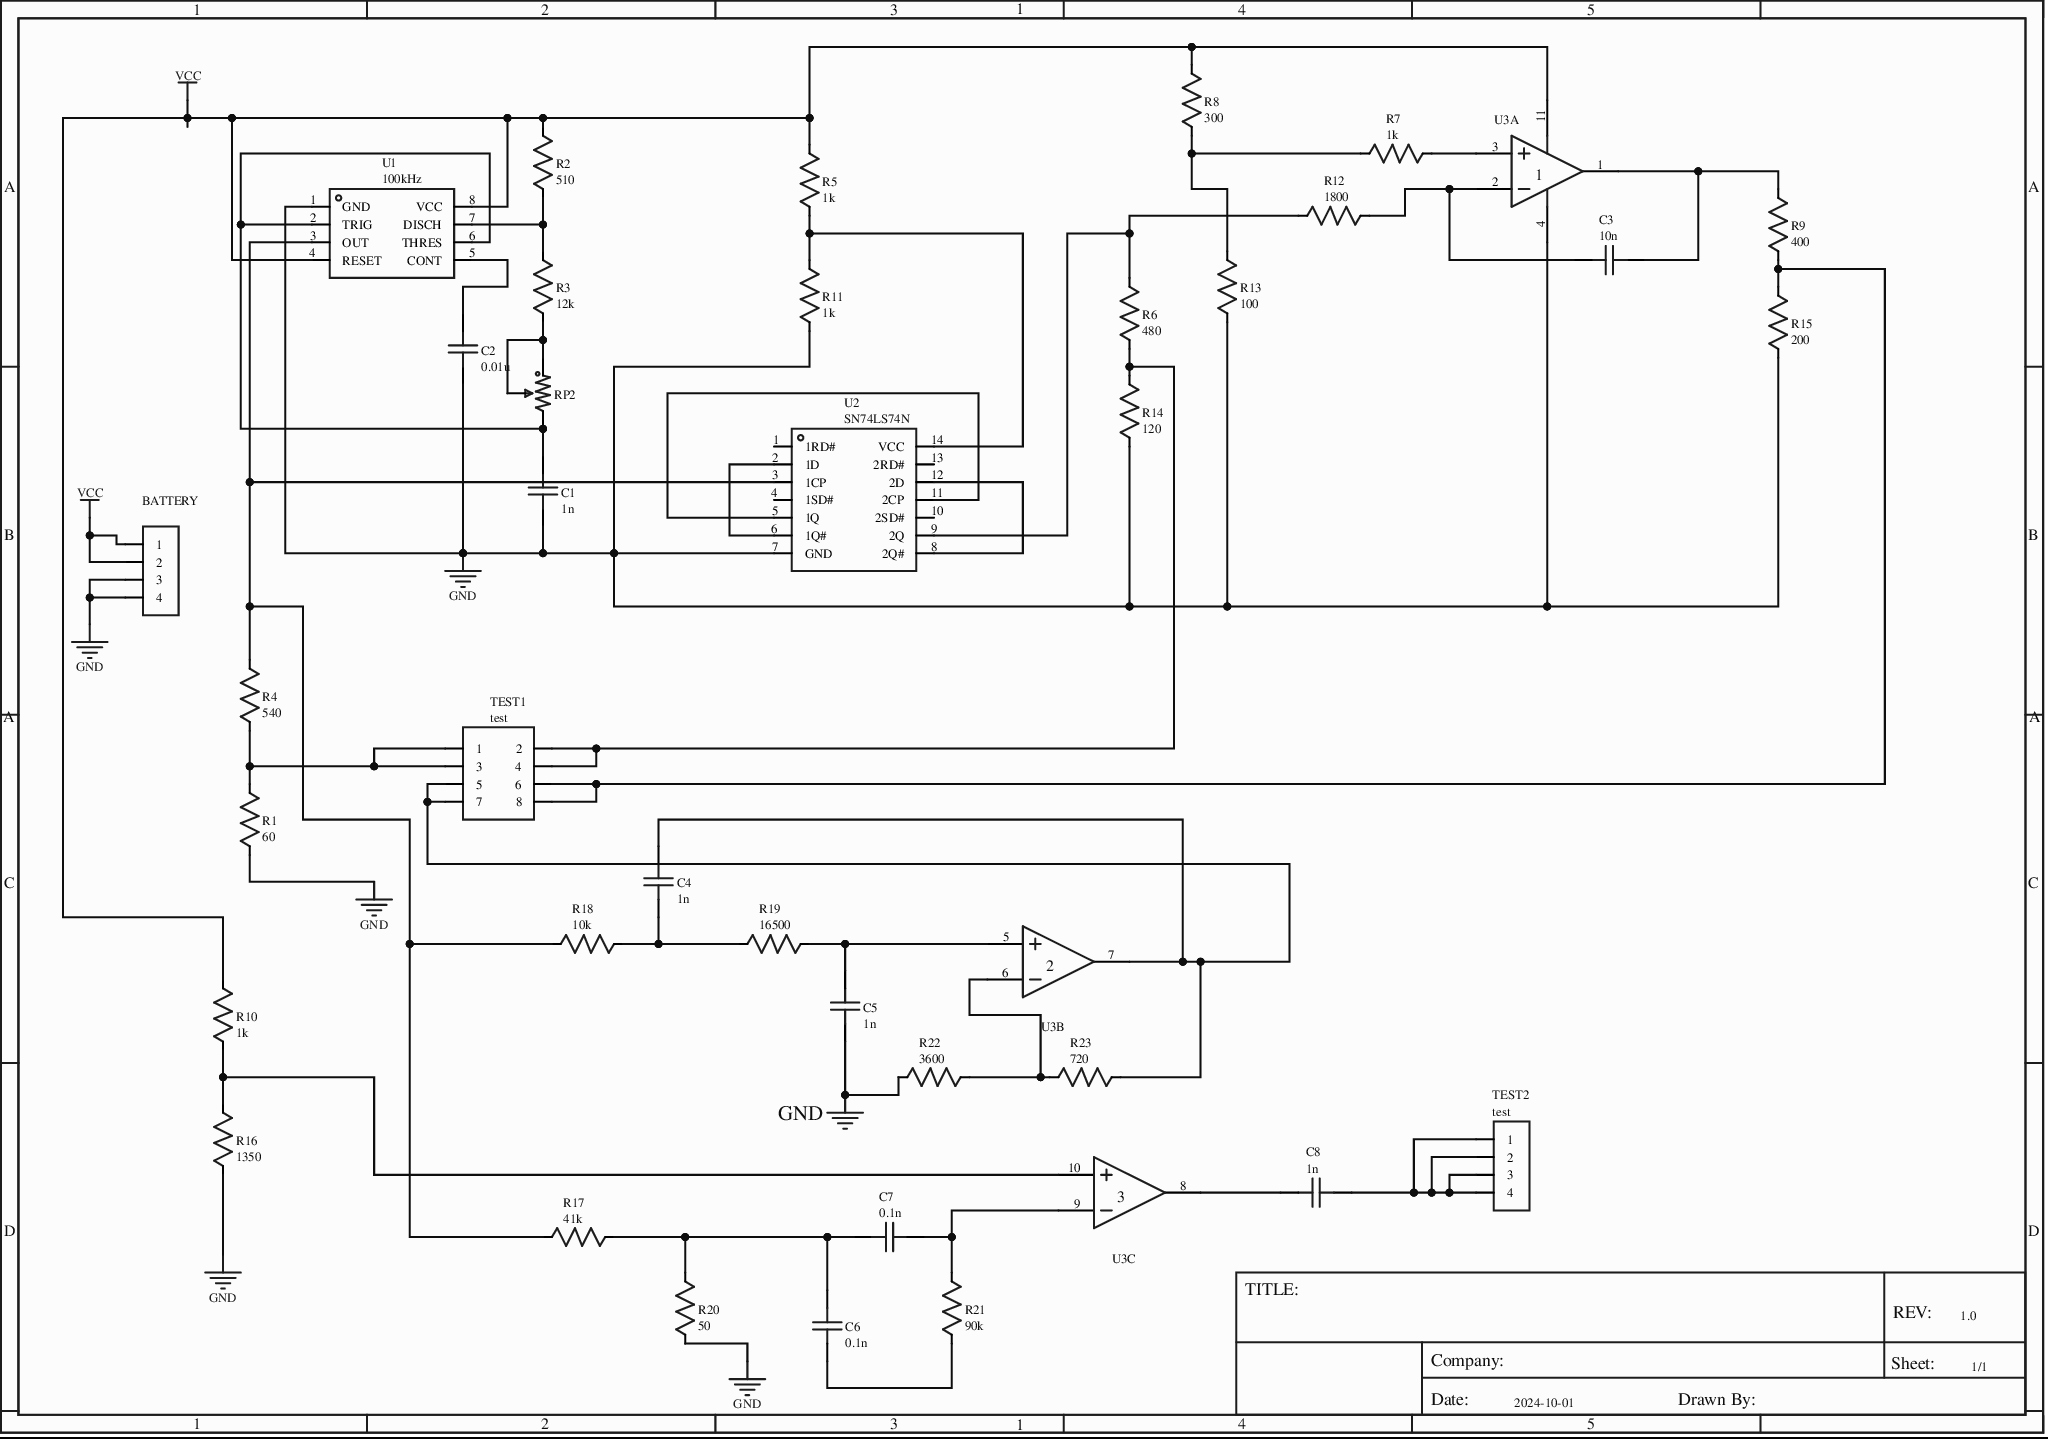
[diagram p0: MISC51938-3.schdoc]
# Altium project MISC51938-2.PrjPcb
1 sheet, 38 parts. Net scope: global (net labels, ports and power ports of the same name join across sheets).
Board file: MISC51938.pcbdoc

## Sheet MISC51938-3.schdoc
size 292 x 204 mm; Name: MISC51938; @Project Name: MISC51938; REV: 1.0; Date: 2024-10-01; Sheet: 1/1

### Parts
BATTERY  HDR-M-2.54_1x4  [HDR-M-2.54_1X4]  (value not drawn)
C1  1n  [RAD-0.1]
C2  0.01u  [RAD-0.1]
C3  10n  [RAD-0.1]
C4  1n  [RAD-0.1]
C5  1n  [RAD-0.1]
C6  0.1n  [RAD-0.1]
C7  0.1n  [RAD-0.1]
C8  1n  [RAD-0.1]
R1  60  [R_AXIAL-0.3]
R2  510  [R_AXIAL-0.3]
R3  12k  [R_AXIAL-0.3]
R4  540  [R_AXIAL-0.3]
R5  1k  [R_AXIAL-0.3]
R6  480  [R_AXIAL-0.3]
R7  1k  [R_AXIAL-0.3]
R8  300  [R_AXIAL-0.3]
R9  400  [R_AXIAL-0.3]
R10  1k  [R_AXIAL-0.3]
R11  1k  [R_AXIAL-0.3]
R12  1800  [R_AXIAL-0.3]
R13  100  [R_AXIAL-0.3]
R14  120  [R_AXIAL-0.3]
R15  200  [R_AXIAL-0.3]
R16  1350  [R_AXIAL-0.3]
R17  41k  [R_AXIAL-0.3]
R18  10k  [R_AXIAL-0.3]
R19  16500  [R_AXIAL-0.3]
R20  50  [R_AXIAL-0.3]
R21  90k  [R_AXIAL-0.3]
R22  3600  [R_AXIAL-0.3]
R23  720  [R_AXIAL-0.3]
RP2  R_3296W_US  [RES-ADJ-TH_3296W]  (value not drawn)
TEST1  test  [HDR-M-2.54_2X4]
TEST2  test  [HDR-M-2.54_1X4]
U1  100kHz  [DIP-8_L9.8-W6.6-P2.54-LS7.6-BL]
U2  SN74LS74N  [DIP-14_L19.1-W6.4-P2.54-LS7.6-BL]
U3  LM324_C5157701  [DIP-14_L18.9-W6.4-P2.54-LS7.6-BL]  (value not drawn)  (parts A,B,C of 3)

### Nets
GND: BATTERY.3 BATTERY.4 C1.1 C2.1 C5.1 R1.1 R11.1 R13.1 R14.1 R15.2 R16.1 R20.2 R22.2 U1.1(GND) U2.7(GND) U3.4(VCC)
VCC: BATTERY.1 BATTERY.2 R2.2 R5.2 R8.2 R10.2 U1.4(RESET) U1.8(VCC) U3.11(GND)
NetC1_2: C1.2 RP2.3 U1.2(TRIG) U1.6(THRES)
NetC2_2: C2.2 U1.5(CONT)
NetC3_1: C3.1 R9.1 U3.1(OUT1)
NetC3_2: C3.2 R12.1 U3.2(IN1-)
NetC4_1: C4.1 R18.1 R19.2
NetC4_2: C4.2 R23.1 TEST1.5 TEST1.7 U3.7(OUT2)
NetC5_2: C5.2 R19.1 U3.5(IN2+)
NetC6_1: C6.1 C7.1 R17.1 R20.1
NetC6_2: C6.2 R21.2
NetC7_2: C7.2 R21.1 U3.9(IN3-)
NetC8_1: C8.1 TEST2.1 TEST2.2 TEST2.3 TEST2.4
NetC8_2: C8.2 U3.8(OUT3)
NetR1_2: R1.2 R4.1 TEST1.1 TEST1.3
NetR2_1: R2.1 R3.2 U1.7(DISCH)
NetR3_1: R3.1 RP2.1 RP2.2
NetR4_2: R4.2 R17.2 R18.2 U1.3(OUT) U2.3(1CP)
NetR5_1: R5.1 R11.2 U2.14(VCC)
NetR6_1: R6.1 R14.2 TEST1.2 TEST1.4
NetR6_2: R6.2 R12.2 U2.9(2Q)
NetR7_1: R7.1 U3.3(IN1+)
NetR7_2: R7.2 R8.1 R13.2
NetR9_2: R9.2 R15.1 TEST1.6 TEST1.8
NetR10_1: R10.1 R16.2 U3.10(IN3+)
NetR22_1: R22.1 R23.2 U3.6(IN2-)
NetU2_2: U2.2(1D) U2.6(1Q#)
NetU2_5: U2.5(1Q) U2.11(2CP)
NetU2_8: U2.8(2Q#) U2.12(2D)

Not connected (* = marked no-connect by the designer): U2 1(1RD#)* 4(1SD#)* 10(2SD#)* 13(2RD#)*

### Notes on the sheet
- GND
- 1
- 2
- 3
- 4
- 5
- A
- B
- C
- D
- TITLE:
- Company:
- Sheet:
- REV:
- 1.0
- 1/1
- Date:
- 2024-10-01
- Drawn By:

### Library data of the parts
BATTERY = HDR-M-2.54_1x4: Convert to PCB: yes; UniqueId: gge182f55f181c338ac; ModelId: cd502121c3eb48dbbf0ecbc8e7ad097f; Origin Footprint: HDR-M-2.54_1X4; Device: HDR-M-2.54_1x4; Symbol: HDR-M-2.54_1x4; Supplier Part: C124378; Supplier: LCSC; Add into BOM: yes; FootprintName: HDR-M-2.54_1X4; ModelName: HDR-M-2.54_1x4
C1 = 1n: Convert to PCB: yes; UniqueId: ggebe2d0743338c48c7; ModelId: 1ae71cde80ce4853a0b9688090c601ad; ModelName: C_RAD-0.1; Origin Footprint: RAD-0.1; Device: 1n; Symbol: 1n; Add into BOM: yes; FootprintName: RAD-0.1
C2 = 0.01u: Convert to PCB: yes; UniqueId: ggec0655fcb97cffe8f; ModelId: 1ae71cde80ce4853a0b9688090c601ad; ModelName: C_RAD-0.1; Origin Footprint: RAD-0.1; Device: 0.01u; Symbol: 0.01u; Add into BOM: yes; FootprintName: RAD-0.1
C3 = 10n: Convert to PCB: yes; UniqueId: gge42024684f1aaf6c8; ModelId: 1ae71cde80ce4853a0b9688090c601ad; ModelName: C_RAD-0.1; Origin Footprint: RAD-0.1; Device: 10n; Symbol: 10n; Add into BOM: yes; FootprintName: RAD-0.1
C4 = 1n: Convert to PCB: yes; UniqueId: gge37dbe484222d80e1; ModelId: 1ae71cde80ce4853a0b9688090c601ad; ModelName: C_RAD-0.1; Origin Footprint: RAD-0.1; Device: 1n; Symbol: 1n; Add into BOM: yes; FootprintName: RAD-0.1
C5 = 1n: Convert to PCB: yes; UniqueId: gge837e8c776d9c40bf; ModelId: 1ae71cde80ce4853a0b9688090c601ad; ModelName: C_RAD-0.1; Origin Footprint: RAD-0.1; Device: 1n; Symbol: 1n; Add into BOM: yes; FootprintName: RAD-0.1
C6 = 0.1n: Convert to PCB: yes; UniqueId: gge8fb21ff73641724b; ModelId: 1ae71cde80ce4853a0b9688090c601ad; ModelName: C_RAD-0.1; Origin Footprint: RAD-0.1; Device: 0.1n; Symbol: 0.1n; Add into BOM: yes; FootprintName: RAD-0.1
C7 = 0.1n: Convert to PCB: yes; UniqueId: gge1a40875608363663; ModelId: 1ae71cde80ce4853a0b9688090c601ad; ModelName: C_RAD-0.1; Origin Footprint: RAD-0.1; Device: 0.1n; Symbol: 0.1n; Add into BOM: yes; FootprintName: RAD-0.1
C8 = 1n: Convert to PCB: yes; UniqueId: gge7d2a8f037e25720b; ModelId: 1ae71cde80ce4853a0b9688090c601ad; ModelName: C_RAD-0.1; Origin Footprint: RAD-0.1; Device: 1n; Symbol: 1n; Add into BOM: yes; FootprintName: RAD-0.1
R1 = 60: Convert to PCB: yes; UniqueId: gge0dfbe59a243fd0c6; ModelId: 3f997efe3b344f2d8e0a2d7f24a0763d; Origin Footprint: R_AXIAL-0.3; Device: 60; Symbol: 60; Add into BOM: yes; FootprintName: R_AXIAL-0.3; ModelName: R_AXIAL-0.3
R2 = 510: Convert to PCB: yes; UniqueId: ggef3c2f23d8da5d148; ModelId: 3f997efe3b344f2d8e0a2d7f24a0763d; Origin Footprint: R_AXIAL-0.3; Device: 510; Symbol: 510; Add into BOM: yes; FootprintName: R_AXIAL-0.3; ModelName: R_AXIAL-0.3
R3 = 12k: Convert to PCB: yes; UniqueId: gge48febd318e5da6c3; ModelId: 3f997efe3b344f2d8e0a2d7f24a0763d; Origin Footprint: R_AXIAL-0.3; Device: 12k; Symbol: 12k; Add into BOM: yes; FootprintName: R_AXIAL-0.3; ModelName: R_AXIAL-0.3
R4 = 540: Convert to PCB: yes; UniqueId: ggefea46ed2f578d9fb; ModelId: 3f997efe3b344f2d8e0a2d7f24a0763d; Origin Footprint: R_AXIAL-0.3; Device: 540; Symbol: 540; Add into BOM: yes; FootprintName: R_AXIAL-0.3; ModelName: R_AXIAL-0.3
R5 = 1k: Convert to PCB: yes; UniqueId: gge40155cd87b47f87c; ModelId: 3f997efe3b344f2d8e0a2d7f24a0763d; Origin Footprint: R_AXIAL-0.3; Device: 1k; Symbol: 1k; Add into BOM: yes; FootprintName: R_AXIAL-0.3; ModelName: R_AXIAL-0.3
R6 = 480: Convert to PCB: yes; UniqueId: ggef7fee3df49b55766; ModelId: 3f997efe3b344f2d8e0a2d7f24a0763d; Origin Footprint: R_AXIAL-0.3; Device: 480; Symbol: 480; Add into BOM: yes; FootprintName: R_AXIAL-0.3; ModelName: R_AXIAL-0.3
R7 = 1k: Convert to PCB: yes; UniqueId: ggef523a0c6794fa5f8; ModelId: 3f997efe3b344f2d8e0a2d7f24a0763d; Origin Footprint: R_AXIAL-0.3; Device: 1k; Symbol: 1k; Add into BOM: yes; FootprintName: R_AXIAL-0.3; ModelName: R_AXIAL-0.3
R8 = 300: Convert to PCB: yes; UniqueId: gge19ed68c85dd61d5f; ModelId: 3f997efe3b344f2d8e0a2d7f24a0763d; Origin Footprint: R_AXIAL-0.3; Device: 300; Symbol: 300; Add into BOM: yes; FootprintName: R_AXIAL-0.3; ModelName: R_AXIAL-0.3
R9 = 400: Convert to PCB: yes; UniqueId: gge2309c8064b6c3153; ModelId: 3f997efe3b344f2d8e0a2d7f24a0763d; Origin Footprint: R_AXIAL-0.3; Device: 400; Symbol: 400; Add into BOM: yes; FootprintName: R_AXIAL-0.3; ModelName: R_AXIAL-0.3
R10 = 1k: Convert to PCB: yes; UniqueId: gge1da9c41bb9003e75; ModelId: 3f997efe3b344f2d8e0a2d7f24a0763d; Origin Footprint: R_AXIAL-0.3; Device: 1k; Symbol: 1k; Add into BOM: yes; FootprintName: R_AXIAL-0.3; ModelName: R_AXIAL-0.3
R11 = 1k: Convert to PCB: yes; UniqueId: ggebda18a44617dddc0; ModelId: 3f997efe3b344f2d8e0a2d7f24a0763d; Origin Footprint: R_AXIAL-0.3; Device: 1k; Symbol: 1k; Add into BOM: yes; FootprintName: R_AXIAL-0.3; ModelName: R_AXIAL-0.3
R12 = 1800: Convert to PCB: yes; UniqueId: ggea9de047fd16be48d; ModelId: 3f997efe3b344f2d8e0a2d7f24a0763d; Origin Footprint: R_AXIAL-0.3; Device: 1800; Symbol: 1800; Add into BOM: yes; FootprintName: R_AXIAL-0.3; ModelName: R_AXIAL-0.3
R13 = 100: Convert to PCB: yes; UniqueId: gge3a1cc0d0732c84e9; ModelId: 3f997efe3b344f2d8e0a2d7f24a0763d; Origin Footprint: R_AXIAL-0.3; Device: 100; Symbol: 100; Add into BOM: yes; FootprintName: R_AXIAL-0.3; ModelName: R_AXIAL-0.3
R14 = 120: Convert to PCB: yes; UniqueId: ggec4de3e0c062074b8; ModelId: 3f997efe3b344f2d8e0a2d7f24a0763d; Origin Footprint: R_AXIAL-0.3; Device: 120; Symbol: 120; Add into BOM: yes; FootprintName: R_AXIAL-0.3; ModelName: R_AXIAL-0.3
R15 = 200: Convert to PCB: yes; UniqueId: gge992ac05409ed4dfa; ModelId: 3f997efe3b344f2d8e0a2d7f24a0763d; Origin Footprint: R_AXIAL-0.3; Device: 200; Symbol: 200; Add into BOM: yes; FootprintName: R_AXIAL-0.3; ModelName: R_AXIAL-0.3
R16 = 1350: Convert to PCB: yes; UniqueId: gge34052e6bc059f6cc; ModelId: 3f997efe3b344f2d8e0a2d7f24a0763d; Origin Footprint: R_AXIAL-0.3; Device: 1350; Symbol: 1350; Add into BOM: yes; FootprintName: R_AXIAL-0.3; ModelName: R_AXIAL-0.3
R17 = 41k: Convert to PCB: yes; UniqueId: ggec6451f7b0751eb53; ModelId: 3f997efe3b344f2d8e0a2d7f24a0763d; Origin Footprint: R_AXIAL-0.3; Device: 41k; Symbol: 41k; Add into BOM: yes; FootprintName: R_AXIAL-0.3; ModelName: R_AXIAL-0.3
R18 = 10k: Convert to PCB: yes; UniqueId: ggeadda2c91ca372ec2; ModelId: 3f997efe3b344f2d8e0a2d7f24a0763d; Origin Footprint: R_AXIAL-0.3; Device: 10k; Symbol: 10k; Add into BOM: yes; FootprintName: R_AXIAL-0.3; ModelName: R_AXIAL-0.3
R19 = 16500: Convert to PCB: yes; UniqueId: gge12cf5a8912aa1a3c; ModelId: 3f997efe3b344f2d8e0a2d7f24a0763d; Origin Footprint: R_AXIAL-0.3; Device: 16500; Symbol: 16500; Add into BOM: yes; FootprintName: R_AXIAL-0.3; ModelName: R_AXIAL-0.3
R20 = 50: Convert to PCB: yes; UniqueId: ggeef11c37f82a57bb4; ModelId: 3f997efe3b344f2d8e0a2d7f24a0763d; Origin Footprint: R_AXIAL-0.3; Device: 50; Symbol: 50; Add into BOM: yes; FootprintName: R_AXIAL-0.3; ModelName: R_AXIAL-0.3
R21 = 90k: Convert to PCB: yes; UniqueId: gge522766d47456ae77; ModelId: 3f997efe3b344f2d8e0a2d7f24a0763d; Origin Footprint: R_AXIAL-0.3; Device: 90k; Symbol: 90k; Add into BOM: yes; FootprintName: R_AXIAL-0.3; ModelName: R_AXIAL-0.3
R22 = 3600: Convert to PCB: yes; UniqueId: gge19f3c2ac4ace3312; ModelId: 3f997efe3b344f2d8e0a2d7f24a0763d; Origin Footprint: R_AXIAL-0.3; Device: 3600; Symbol: 3600; Add into BOM: yes; FootprintName: R_AXIAL-0.3; ModelName: R_AXIAL-0.3
R23 = 720: Convert to PCB: yes; UniqueId: gge608eda8aeb79ff7f; ModelId: 3f997efe3b344f2d8e0a2d7f24a0763d; Origin Footprint: R_AXIAL-0.3; Device: 720; Symbol: 720; Add into BOM: yes; FootprintName: R_AXIAL-0.3; ModelName: R_AXIAL-0.3
RP2 = R_3296W_US: value(Ω): 10K; Convert to PCB: yes; UniqueId: gge5340c3f8fc1e4fdc; ModelId: 3664f7b541aa4725a8b6d3b7a961f078; Origin Footprint: RES-ADJ-TH_3296W; Device: R_3296W_US; Symbol: R_3296W_US; Supplier: LCSC; Add into BOM: yes; FootprintName: RES-ADJ-TH_3296W; ModelName: RES-ADJ-TH_3296W
TEST1 = test: Convert to PCB: yes; UniqueId: ggeb8db4d18d316af96; ModelId: a46776abaaac4775bf058ba5fc9d0d80; Origin Footprint: HDR-M-2.54_2X4; Device: test; Symbol: test; Supplier Part: C58363; Supplier: LCSC; Add into BOM: yes; FootprintName: HDR-M-2.54_2X4; ModelName: HDR-M-2.54_2x4
TEST2 = test: Convert to PCB: yes; UniqueId: gge0dde4e04bc7630b6; ModelId: cd502121c3eb48dbbf0ecbc8e7ad097f; Origin Footprint: HDR-M-2.54_1X4; Device: test; Symbol: test; Supplier Part: C124378; Supplier: LCSC; Add into BOM: yes; FootprintName: HDR-M-2.54_1X4; ModelName: HDR-M-2.54_1x4
U1 = 100kHz: Manufacturer: TI(德州仪器); Manufacturer Part: NE555P; Convert to PCB: yes; UniqueId: gge9076eb39313fc52a; ModelId: db2af726fcec488f8bf8e467aca974b3; ModelName: DIP-8_L9.8-W6.6-H3.5-LS7.62-P2.54; Origin Footprint: DIP-8_L9.8-W6.6-P2.54-LS7.6-BL; Device: 100kHz; Symbol: 100kHz; Supplier: LCSC; Supplier Part: C46749; JLCPCB Part Class: Extended Part; Add into BOM: yes; FootprintName: DIP-8_L9.8-W6.6-P2.54-LS7.6-BL
U2 = SN74LS74N: Manufacturer: LX(灵星芯微); Convert to PCB: yes; UniqueId: gge7974bd9af496d1f7; ModelId: 4fb82330961949e587245d1f3ebad69c; Origin Footprint: DIP-14_L19.1-W6.4-P2.54-LS7.6-BL; Device: SN74LS74N; Symbol: SN74LS74N; Supplier: LCSC; Supplier Part: C22466308; Manufacturer Part: SN74LS74N; JLCPCB Part Class: Extended Part; Add into BOM: yes; FootprintName: DIP-14_L19.1-W6.4-P2.54-LS7.6-BL; ModelName: DIP-14_L19.1-W6.4-P2.54-LS7.6-BL
U3 = LM324_C5157701: Manufacturer: Gcore(扬州国芯); Manufacturer Part: LM324; Convert to PCB: yes; UniqueId: ggea0a54a629d26c036; ModelId: 6184deb591d44bb6a4993f827f8048e2; Origin Footprint: DIP-14_L18.9-W6.4-P2.54-LS7.6-BL; Device: LM324_C5157701; Symbol: LM324_C5157701; Supplier: LCSC; Supplier Part: C5157701; JLCPCB Part Class: Extended Part; Add into BOM: yes; FootprintName: DIP-14_L18.9-W6.4-P2.54-LS7.6-BL; ModelName: DIP-14_L18.9-W6.4-P2.54-LS7.6-BL